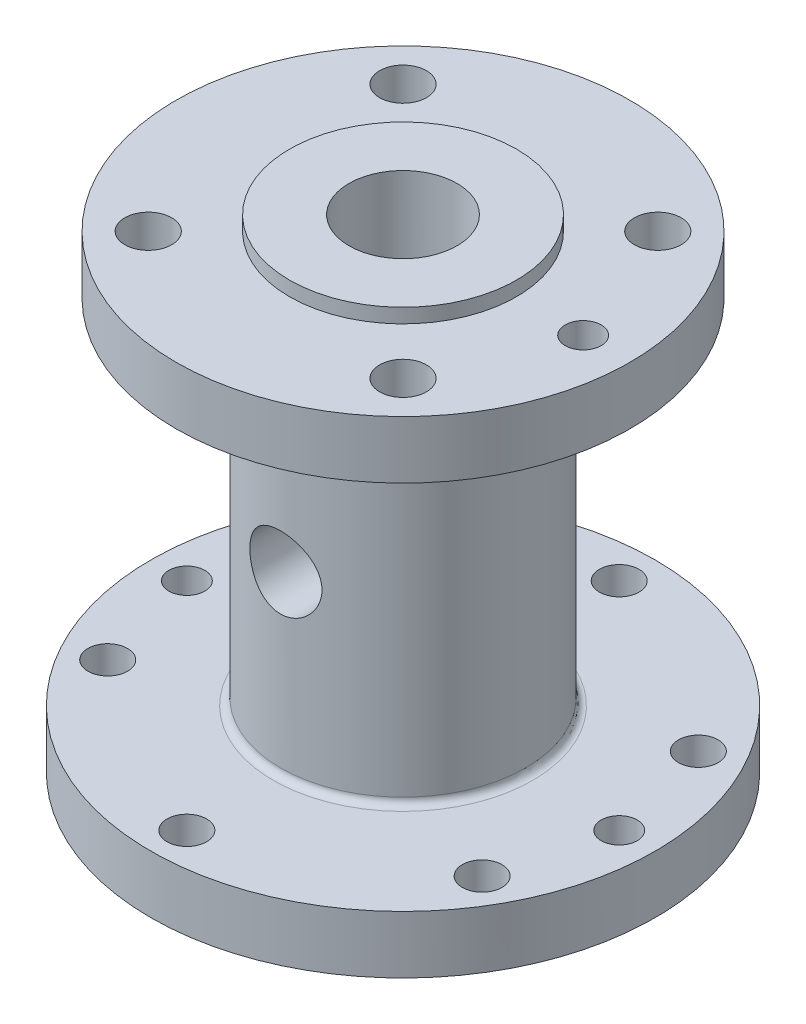
from build123d import *

# Parameters (mm, degrees)
SKETCH_1_R             = 35
EXTRUDE_1_DEPTH        = 32.5
SKETCH_3_W             = 18
SKETCH_3_H             = 49
FILLET_1_R             = 1
SKETCH_6_R             = 7.5
CUT_EXTRUDE_3_DEPTH    = 82.700673192
HOLE_WIZARD_M5_1_D     = 5.5
HOLE_WIZARD_M5_1_DEPTH = 15
HOLE_WIZARD_M5_1_TIP   = 1.652366702
F_5_0MM_1_D            = 5
F_5_0MM_1_DEPTH        = 10
F_5_0MM_1_TIP          = 1.502151548
SKETCH_11_R            = 5
CUT_EXTRUDE_4_DEPTH    = 30
SKETCH_15_OUTSIDE_W    = 95.686
SKETCH_15_OUTSIDE_H    = 95.686
SKETCH_15_OUTSIDE_R    = 31.5
CUT_EXTRUDE_6_DEPTH    = 8
EXTRUDE_START          = 2
SKETCH_16_R            = 15.75
SKETCH_16_R_2          = 7.5
EXTRUDE_2_DEPTH        = 2
SKETCH_17_R            = 3.25
SKETCH_17_R_2          = 2.5
CUT_EXTRUDE_7_DEPTH    = 8


with BuildPart() as part:
    # 草图1 → 凸台-拉伸1 (new, symmetric)
    with BuildSketch(Plane(origin=(0, 0, 0), x_dir=(1, 0, 0), z_dir=(0, 1, 0))):
        with Locations(Location((0, 0, 0), (0, 0, 270))):
            Circle(SKETCH_1_R)
    extrude(amount=EXTRUDE_1_DEPTH, both=True)

    # 草图3 → 切除-旋转1 (revolve, cut)
    with BuildSketch(Plane.XY, mode=Mode.PRIVATE) as cut_revolve_1_sk:
        with Locations((26, 0)):
            Rectangle(SKETCH_3_W, SKETCH_3_H)
    revolve(cut_revolve_1_sk.sketch.rotate(Axis((0, 0, 0), (0, 1, 0)), 90), axis=Axis((0, 0, 0), (0, 1, 0)), mode=Mode.SUBTRACT)

    # 圆角1
    fillet_1_edges = [part.edges().sort_by_distance(p)[0] for p in [
        (0, 24.5, 17),
        (0, -24.5, 17),
    ]]
    fillet(fillet_1_edges, radius=FILLET_1_R)

    # 草图6 → 切除-拉伸3 (cut, through all)
    with BuildSketch(Plane(origin=(0, 32.5, 0), x_dir=(1, 0, 0), z_dir=(0, 1, 0))):
        with Locations(Location((0, 0, 0), (0, 0, 180))):
            Circle(SKETCH_6_R)
    extrude(amount=-CUT_EXTRUDE_3_DEPTH, mode=Mode.SUBTRACT)

    # M5 间隙孔1
    with Locations(Plane(origin=(0, -32.5, 0), x_dir=(-1, 0, 0), z_dir=(0, -1, 0))):
        with Locations((0, -30), (-25.980762114, -15), (-25.980762114, 15), (0, 30), (25.980762114, 15), (25.980762114, -15)):
            Hole(HOLE_WIZARD_M5_1_D / 2, depth=HOLE_WIZARD_M5_1_DEPTH)
            with Locations((0, 0, -(HOLE_WIZARD_M5_1_DEPTH + HOLE_WIZARD_M5_1_TIP / 2))):  # 118° drill point
                Cone(0, HOLE_WIZARD_M5_1_D / 2, HOLE_WIZARD_M5_1_TIP, mode=Mode.SUBTRACT)

    # Ø5.0mm 暗销孔1
    with Locations(Plane(origin=(0, -32.5, 0), x_dir=(-1, 0, 0), z_dir=(0, -1, 0))):
        with Locations((-30, 0), (30, 0)):
            Hole(F_5_0MM_1_D / 2, depth=F_5_0MM_1_DEPTH)
            with Locations((0, 0, -(F_5_0MM_1_DEPTH + F_5_0MM_1_TIP / 2))):  # 118° drill point
                Cone(0, F_5_0MM_1_D / 2, F_5_0MM_1_TIP, mode=Mode.SUBTRACT)

    # 草图11 → 切除-拉伸4 (cut, symmetric)
    with BuildSketch(Plane.XY):
        Circle(SKETCH_11_R)
    extrude(amount=CUT_EXTRUDE_4_DEPTH, both=True, mode=Mode.SUBTRACT)

    # 草图15 outside → 切除-拉伸6 (cut)
    with BuildSketch(Plane(origin=(0, 32.5, 0), x_dir=(1, 0, 0), z_dir=(0, 1, 0))):
        Rectangle(SKETCH_15_OUTSIDE_W, SKETCH_15_OUTSIDE_H)
        with Locations(Location((0, 0, 0), (0, 0, 270))):
            Circle(SKETCH_15_OUTSIDE_R, mode=Mode.SUBTRACT)
    extrude(amount=-CUT_EXTRUDE_6_DEPTH, mode=Mode.SUBTRACT)

    # 草图16 → 凸台-拉伸2 (add)
    with BuildSketch(Plane(origin=(0, 32.5, 0), x_dir=(1, 0, 0), z_dir=(0, 1, 0)).offset(EXTRUDE_START)):
        with Locations(Location((0, 0, 0), (0, 0, 270))):
            Circle(SKETCH_16_R)
        with Locations(Location((0, 0, 0), (0, 0, 180))):
            Circle(SKETCH_16_R_2, mode=Mode.SUBTRACT)
    extrude(amount=-EXTRUDE_2_DEPTH)

    # 草图17 → 切除-拉伸7 (cut)
    with BuildSketch(Plane(origin=(0, 32.5, 0), x_dir=(1, 0, 0), z_dir=(0, 1, 0))):
        with Locations(Location((-17.67766953, -17.67766953, 0), (0, 0, 270))):
            Circle(SKETCH_17_R)
        with Locations(Location((-17.67766953, 17.67766953, 0), (0, 0, 270))):
            Circle(SKETCH_17_R)
        with Locations(Location((17.67766953, 17.67766953, 0), (0, 0, 270))):
            Circle(SKETCH_17_R)
        with Locations(Location((17.67766953, -17.67766953, 0), (0, 0, 270))):
            Circle(SKETCH_17_R)
        with Locations(Location((25, 0, 0), (0, 0, 270))):
            Circle(SKETCH_17_R_2)
    extrude(amount=-CUT_EXTRUDE_7_DEPTH, mode=Mode.SUBTRACT)


solid = part.part
